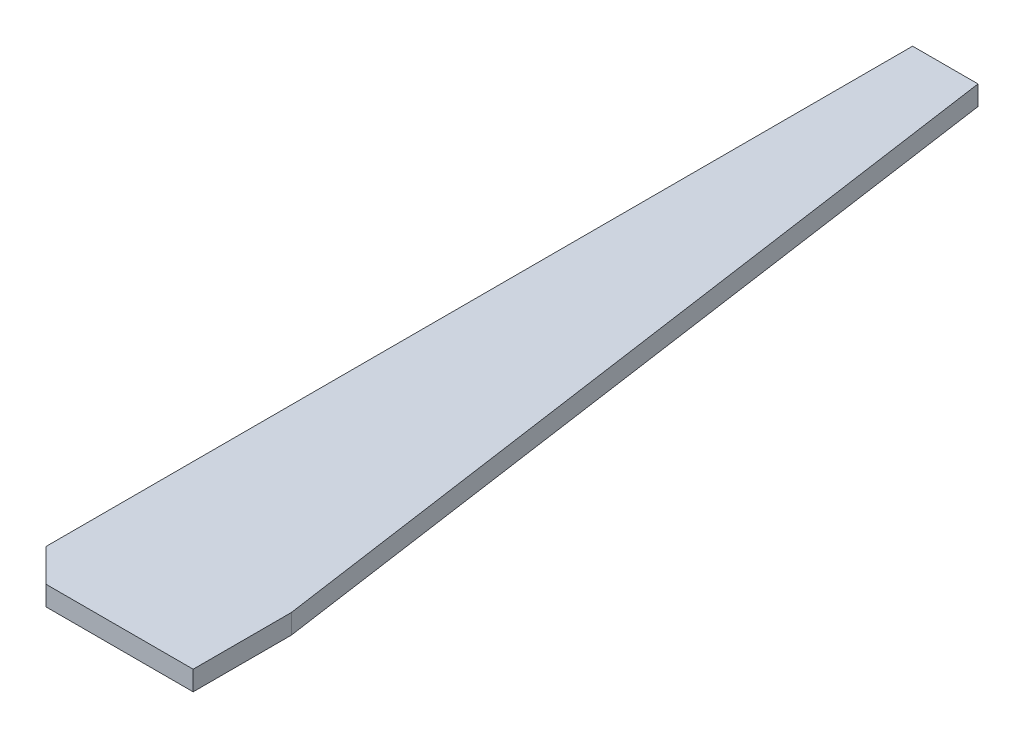
SolidWorks part; units mm, degrees
material "Q235B"
ref_plane "Front Plane" through (0, 0, 0) normal (0, 0, 1) x (1, 0, 0)
ref_plane "Top Plane" through (0, 0, 0) normal (0, 1, 0) x (1, 0, 0)
ref_plane "Right Plane" through (0, 0, 0) normal (1, 0, 0) x (0, 0, -1)
sketch "Sketch1" plane through (0, 0, 0) normal (0, 1, 0) x (1, 0, 0)
  line L10 (0, 0) -> (-20, 20) construction
  line L11 (-20, 20) -> (-20, 550)
  line L13 (-20, 550) -> (20, 550)
  line L14 (20, 550) -> (90, 60)
  line L15 (90, 60) -> (90, 0)
  line L16 (90, 0) -> (0, 0)
  line L17 (-20, 20) -> (-20, 0)
  line L18 (-20, 0) -> (0, 0)
  dimension "D1" = 20
  dimension "D5" = 60
  dimension "D8" = 40
  dimension "D2" = 20
  dimension "D4" = 110
  dimension "D7" = 550
extrude "Boss-Extrude1" add sketch "Sketch1" along normal mid plane 12
chamfer "Chamfer1" distance 20 angle 45 1 edges at (-20, 0, 0)
